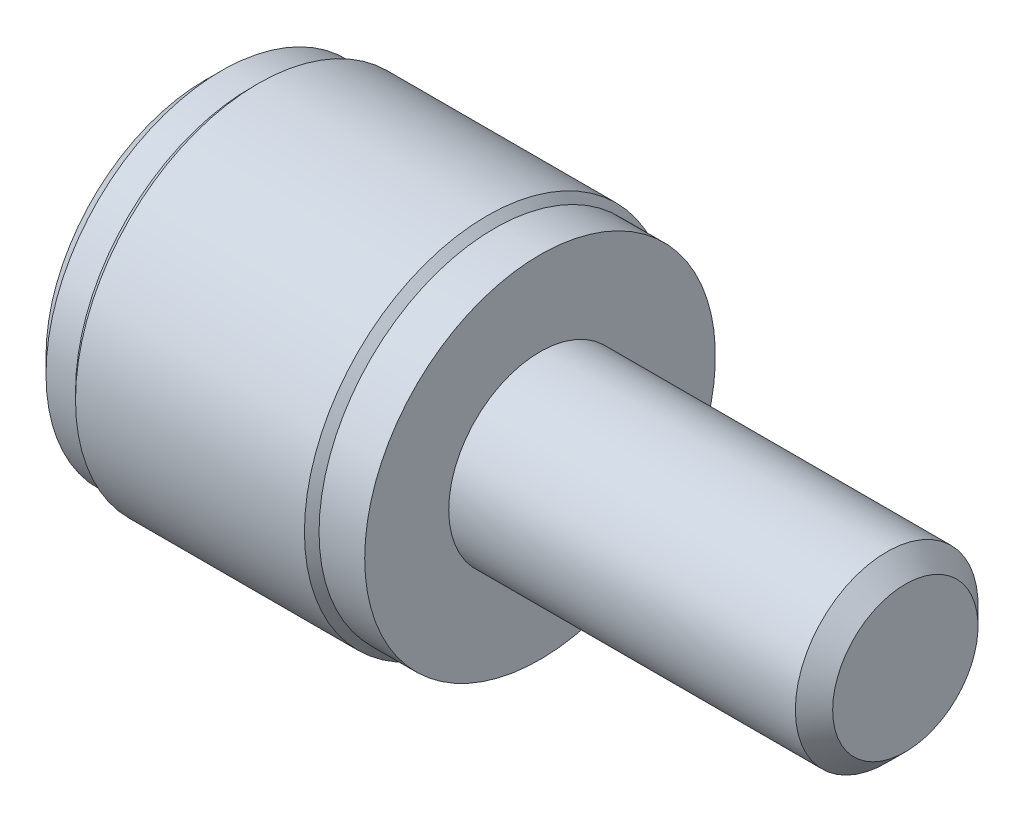
SolidWorks part; units mm, degrees
material "普通碳钢"
ref_plane "Front Plane" through (0, 0, 0) normal (0, 0, 1) x (1, 0, 0)
ref_plane "Top Plane" through (0, 0, 0) normal (0, 1, 0) x (1, 0, 0)
ref_plane "Right Plane" through (0, 0, 0) normal (1, 0, 0) x (0, 0, -1)
sketch "Sketch1" plane through (0, 0, 0) normal (0, 0, 1) x (1, 0, 0)
  line L0 (-5.5, 0) -> (-5.5, 2.6148)
  line L1 (-5.5, 2.6148) -> (-5.2348, 2.88)
  line L2 (-5.2348, 2.88) -> (-4.75, 2.88)
  line L3 (-4.75, 2.88) -> (-4.63, 3)
  line L4 (-4.63, 3) -> (-0.87, 3)
  line L5 (-0.87, 3) -> (-0.75, 2.88)
  line L6 (-0.75, 2.88) -> (0, 2.88)
  line L7 (0, 2.88) -> (0, 1.5)
  line L8 (0, 1.5) -> (5.6935, 1.5)
  line L9 (5.6935, 1.5) -> (6, 1.1935)
  line L10 (6, 1.1935) -> (6, 0)
  line L11 (6, 0) -> (-5.5, 0)
  line L12 (6, 0) -> (-5.5, 0) construction
revolve "Revolve1" add sketch "Sketch1" angle 360 about L12
cosmetic thread "Cosmetic Thread1" parameters "D1"=3, "D2"=2.387
sketch "Sketch2" plane through (0, 0, 0) normal (0, 0, 1) x (1, 0, 0)
  line L0 (-5.5, 0) -> (-5.5, 0.91)
  line L1 (-5.5, 0.91) -> (-5.11, 0.52)
  line L2 (-5.11, 0.52) -> (-3.0502, 0.52)
  line L3 (-3.0502, 0.52) -> (-2.75, 0)
  line L4 (-2.75, 0) -> (-5.5, 0)
  line L5 (-2.75, 0) -> (-5.5, 0) construction
revolve "Cut-Revolve1" cut sketch "Sketch2" angle 360 about L5
ref_plane "Plane1" through (-5.5, 0, 0) normal (1, 0, 0) x (0, 0, -1)
sketch "Sketch3" plane through (-5.5, 0, 0) normal (1, 0, 0) x (0, 0, -1)
  line L0 (-0.65, 0.3753) -> (-0.65, -0.3753)
  line L1 (-0.65, -0.3753) -> (0, -0.7506)
  line L2 (0, -0.7506) -> (0.65, -0.3753)
  line L3 (0.65, -0.3753) -> (0.65, 0.3753)
  line L4 (0.65, 0.3753) -> (0, 0.7506)
  line L5 (0, 0.7506) -> (-0.65, 0.3753)
extrude "Cut-Extrude1" cut sketch "Sketch3" along normal blind 1.8333
